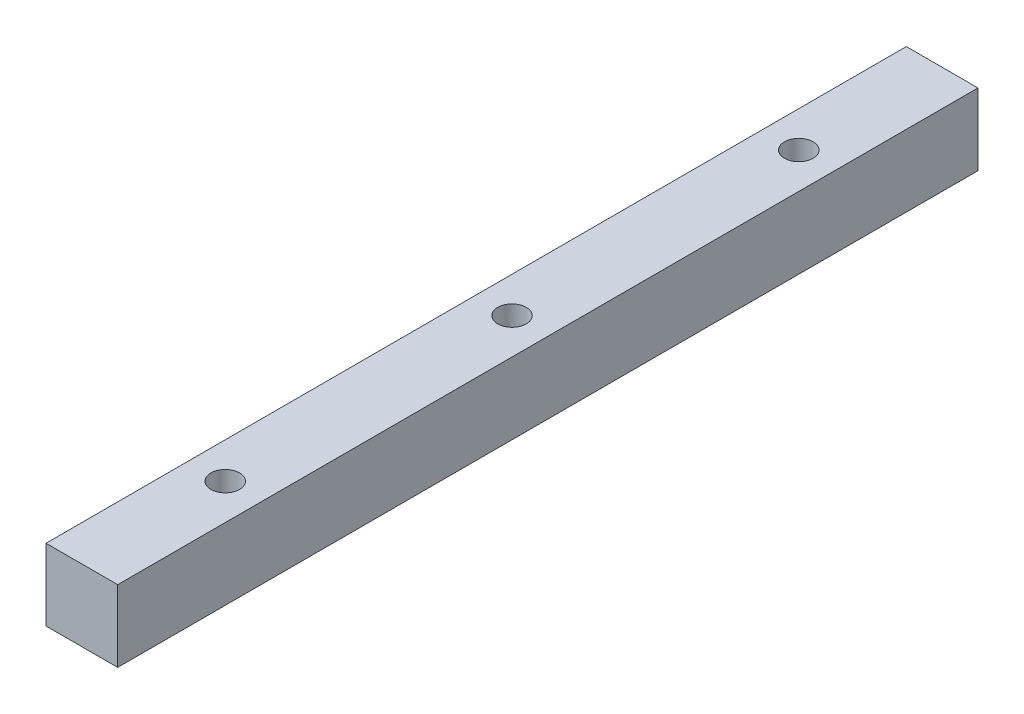
SolidWorks part; units mm, degrees
material "普通碳钢"
ref_plane "前视基准面" through (0, 0, 0) normal (0, 0, 1) x (1, 0, 0)
ref_plane "上视基准面" through (0, 0, 0) normal (0, 1, 0) x (1, 0, 0)
ref_plane "右视基准面" through (0, 0, 0) normal (1, 0, 0) x (0, 0, -1)
sketch "草图1" plane through (0, 0, 0) normal (0, 0, 1) x (1, 0, 0)
  line L1 (-7.5, 7.5) -> (7.5, 7.5)
  line L2 (-7.5, 7.5) -> (-7.5, -7.5)
  line L3 (-7.5, -7.5) -> (7.5, -7.5)
  line L4 (7.5, 7.5) -> (7.5, -7.5)
  line L5 (-7.5, 7.5) -> (7.5, -7.5) construction
  line L6 (-7.5, -7.5) -> (7.5, 7.5) construction
  point P0 (0, 0)
  dimension "D1" = 15
  dimension "D2" = 15
extrude "凸台-拉伸1" add sketch "草图1" along normal mid plane 180
sketch "草图2" plane through (0, 7.5, 0) normal (0, 1, 0) x (1, 0, 0)
  line L0 (0, -60) -> (0, -90) construction
  line L1 (7.5, -90) -> (-7.5, -90) construction
  circle A0 centre (0, -60) radius 3
  dimension "D2" = 6
  dimension "D1" = 30
extrude "切除-拉伸1" cut sketch "草图2" against normal blind 4.5
sketch "草图3" plane through (0, 7.5, 0) normal (0, 1, 0) x (1, 0, 0)
  circle A0 centre (0, -60) radius 2
  dimension "D1" = 4
extrude "切除-拉伸2" cut sketch "草图3" against normal through all
pattern_linear "阵列(线性)1" count 4 spacing 60 along (0, 0, -1) of "切除-拉伸1", "切除-拉伸2"
